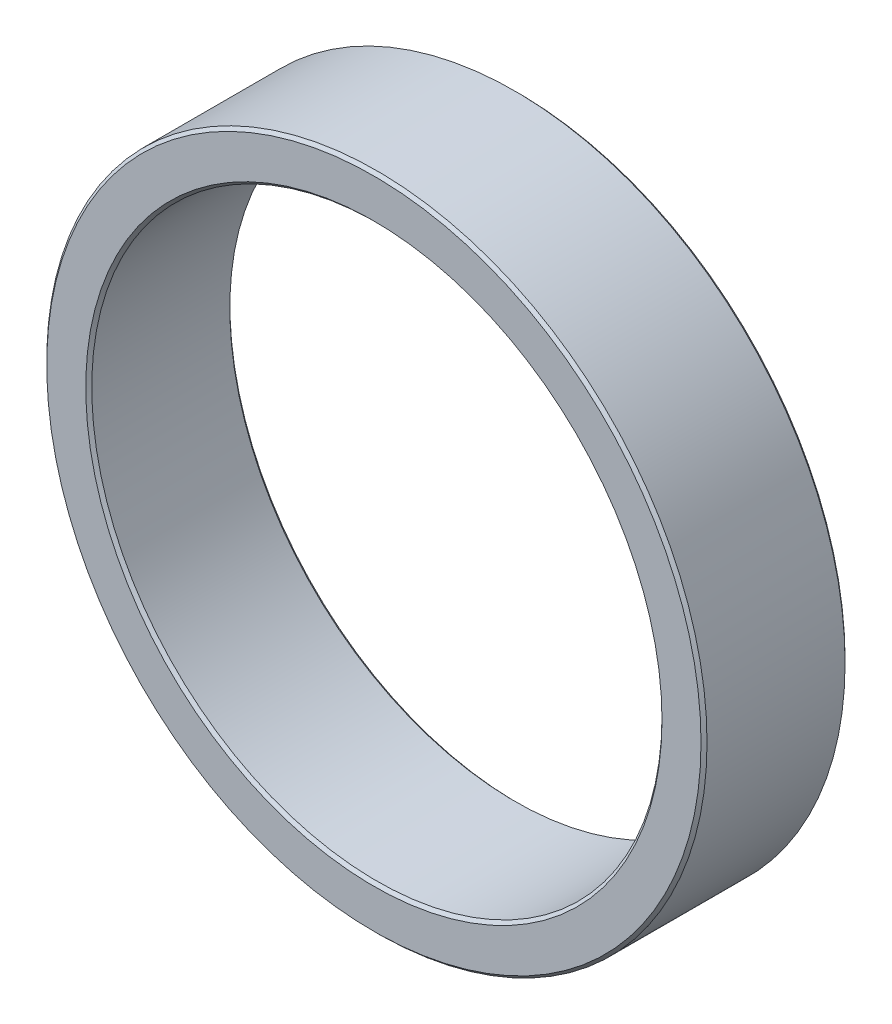
SolidWorks part; units mm, degrees
ref_plane "Front Plane" through (0, 0, 0) normal (0, 0, 1) x (1, 0, 0)
ref_plane "Top Plane" through (0, 0, 0) normal (0, 1, 0) x (1, 0, 0)
ref_plane "Right Plane" through (0, 0, 0) normal (1, 0, 0) x (0, 0, -1)
sketch "Sketch1" plane through (0, 0, 0) normal (0, 0, 1) x (1, 0, 0)
  circle A0 centre (0, 0) radius 55
  circle A1 centre (0, 0) radius 47.5
  dimension "D1" = 110
  dimension "D2" = 95
extrude "Boss-Extrude1" add sketch "Sketch1" along normal blind 24
chamfer "Chamfer1" distance 0.5 angle 45 4 edges at (47.5, 0, 0) (55, 0, 0) (47.5, 0, 24) (55, 0, 24)
